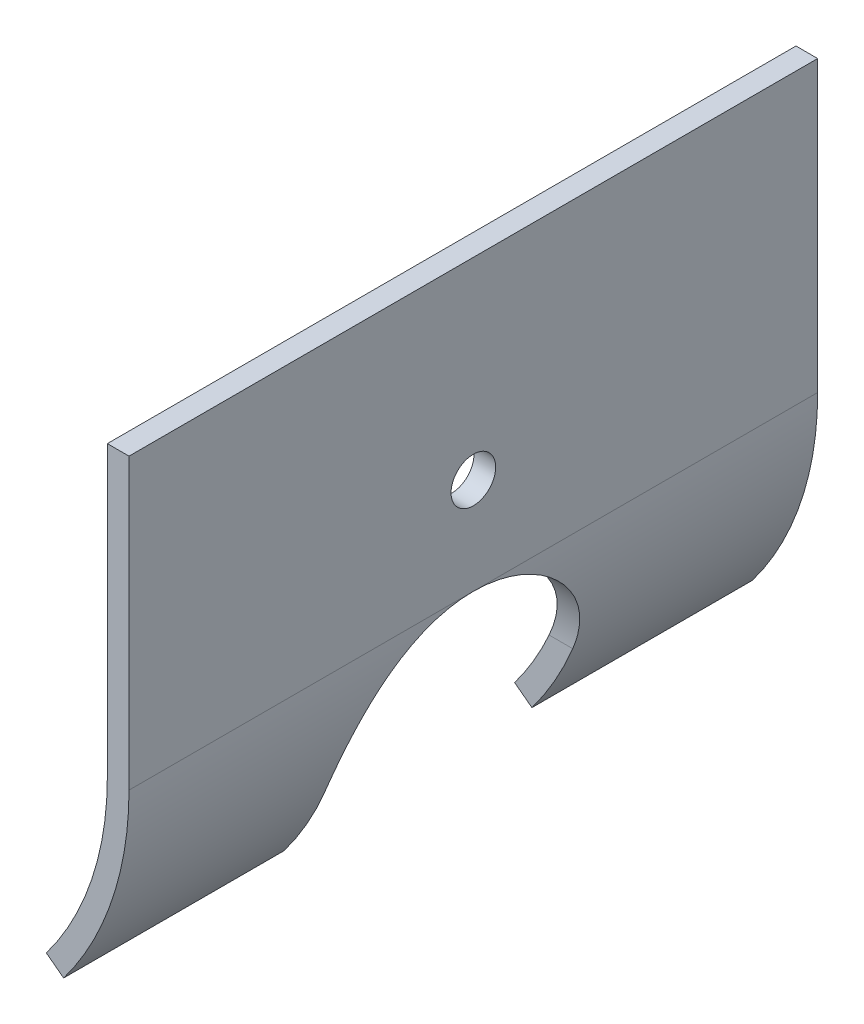
SolidWorks part; units mm, degrees
material "普通碳钢"
ref_plane "Front Plane" through (0, 0, 0) normal (0, 0, 1) x (1, 0, 0)
ref_plane "Top Plane" through (0, 0, 0) normal (0, 1, 0) x (1, 0, 0)
ref_plane "Right Plane" through (0, 0, 0) normal (1, 0, 0) x (0, 0, -1)
sketch "Sketch1" plane through (0, 0, 0) normal (0, 0, 1) x (1, 0, 0)
  line L0 (-149.7, -44.45) -> (81.4749, -44.45) construction
  line L1 (-10, 88.9) -> (0, 88.9)
  line L2 (-10, 88.9) -> (-10, -44.45)
  line L3 (-30.1443, -134.5417) -> (-38.1306, -128.5236)
  line L4 (0, 88.9) -> (0, -44.45)
  line L5 (-149.7, -44.45) -> (47.8834, -193.3398) construction
  arc A0 (-38.1306, -128.5236) -> (-10, -44.45) centre (-149.7, -44.45) ccw
  arc A1 (-30.1443, -134.5417) -> (0, -44.45) centre (-149.7, -44.45) ccw
  dimension "D5" = 139.7
  dimension "D1" = 10
  dimension "D2" = 10
  dimension "D3" = 133.35
  dimension "D4" = 88.9
  dimension "D6" = 37
extrude "Boss-Extrude1" add sketch "Sketch1" along normal mid plane 317.5
sketch "Sketch4" plane through (0, 0, 0) normal (1, 0, 0) x (0, 0, -1)
  line L0 (0, 159.9638) -> (0, -324.9579) construction
  line L1 (-57.15, -101.6) -> (-57.15, -134.5417)
  line L2 (-158.75, -134.5417) -> (158.75, -134.5417) construction
  line L3 (-57.15, -134.5417) -> (57.15, -134.5417)
  line L4 (57.15, -134.5417) -> (57.15, -101.6)
  line L5 (-158.75, -44.45) -> (158.75, -44.45) construction
  circle A0 centre (0, 0) radius 10.287
  arc A1 (57.15, -101.6) -> (-57.15, -101.6) centre (0, -101.6) ccw
  dimension "D1" = 20.574
  dimension "D2" = 114.3
extrude "Cut-Extrude1" cut sketch "Sketch4" against normal mid plane 368.3
